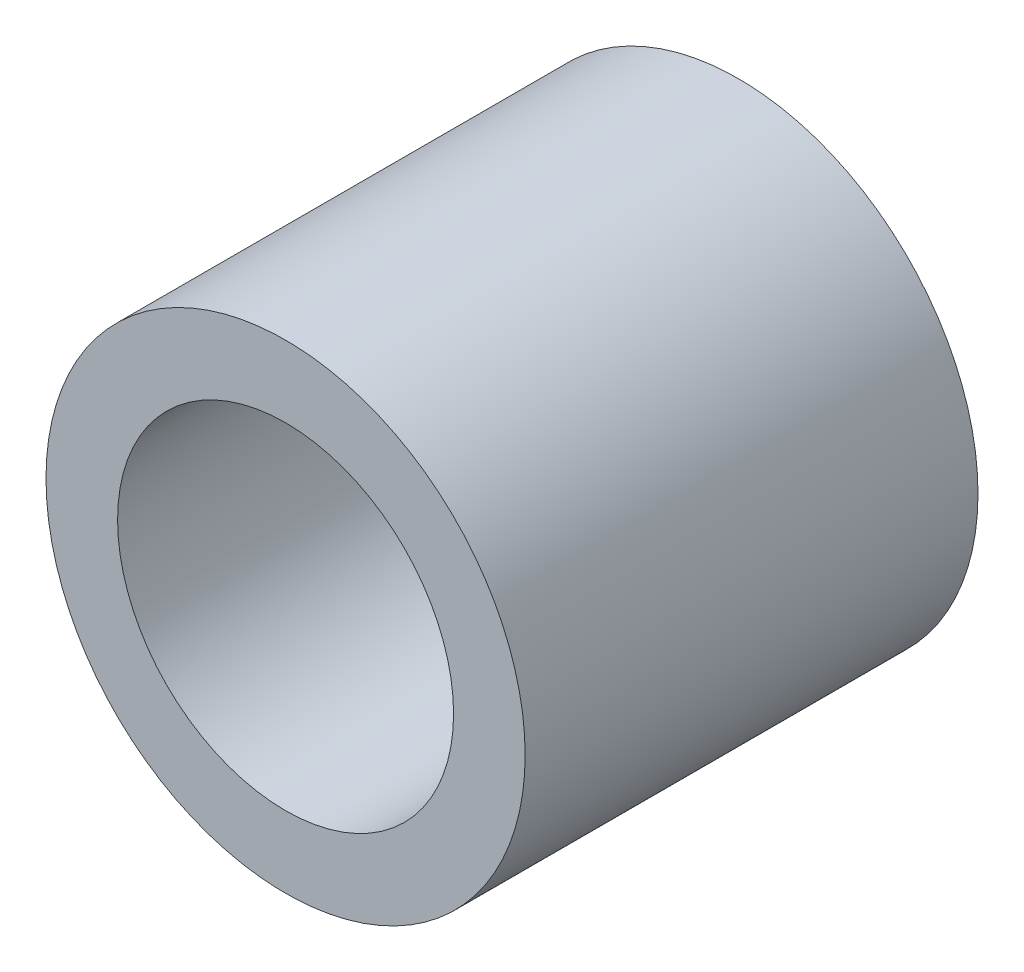
SolidWorks part; units mm, degrees
ref_plane "前视基准面" through (0, 0, 0) normal (0, 0, 1) x (1, 0, 0)
ref_plane "上视基准面" through (0, 0, 0) normal (0, 1, 0) x (1, 0, 0)
ref_plane "右视基准面" through (0, 0, 0) normal (1, 0, 0) x (0, 0, -1)
sketch "草图1" plane through (0, 0, 0) normal (0, 0, 1) x (1, 0, 0)
  circle A0 centre (0, 0) radius 1.15
  circle A1 centre (0, 0) radius 1.64
  dimension "D1" = 2.3
  dimension "D2" = 3.28
extrude "凸台-拉伸1" add sketch "草图1" along normal blind 3.1
